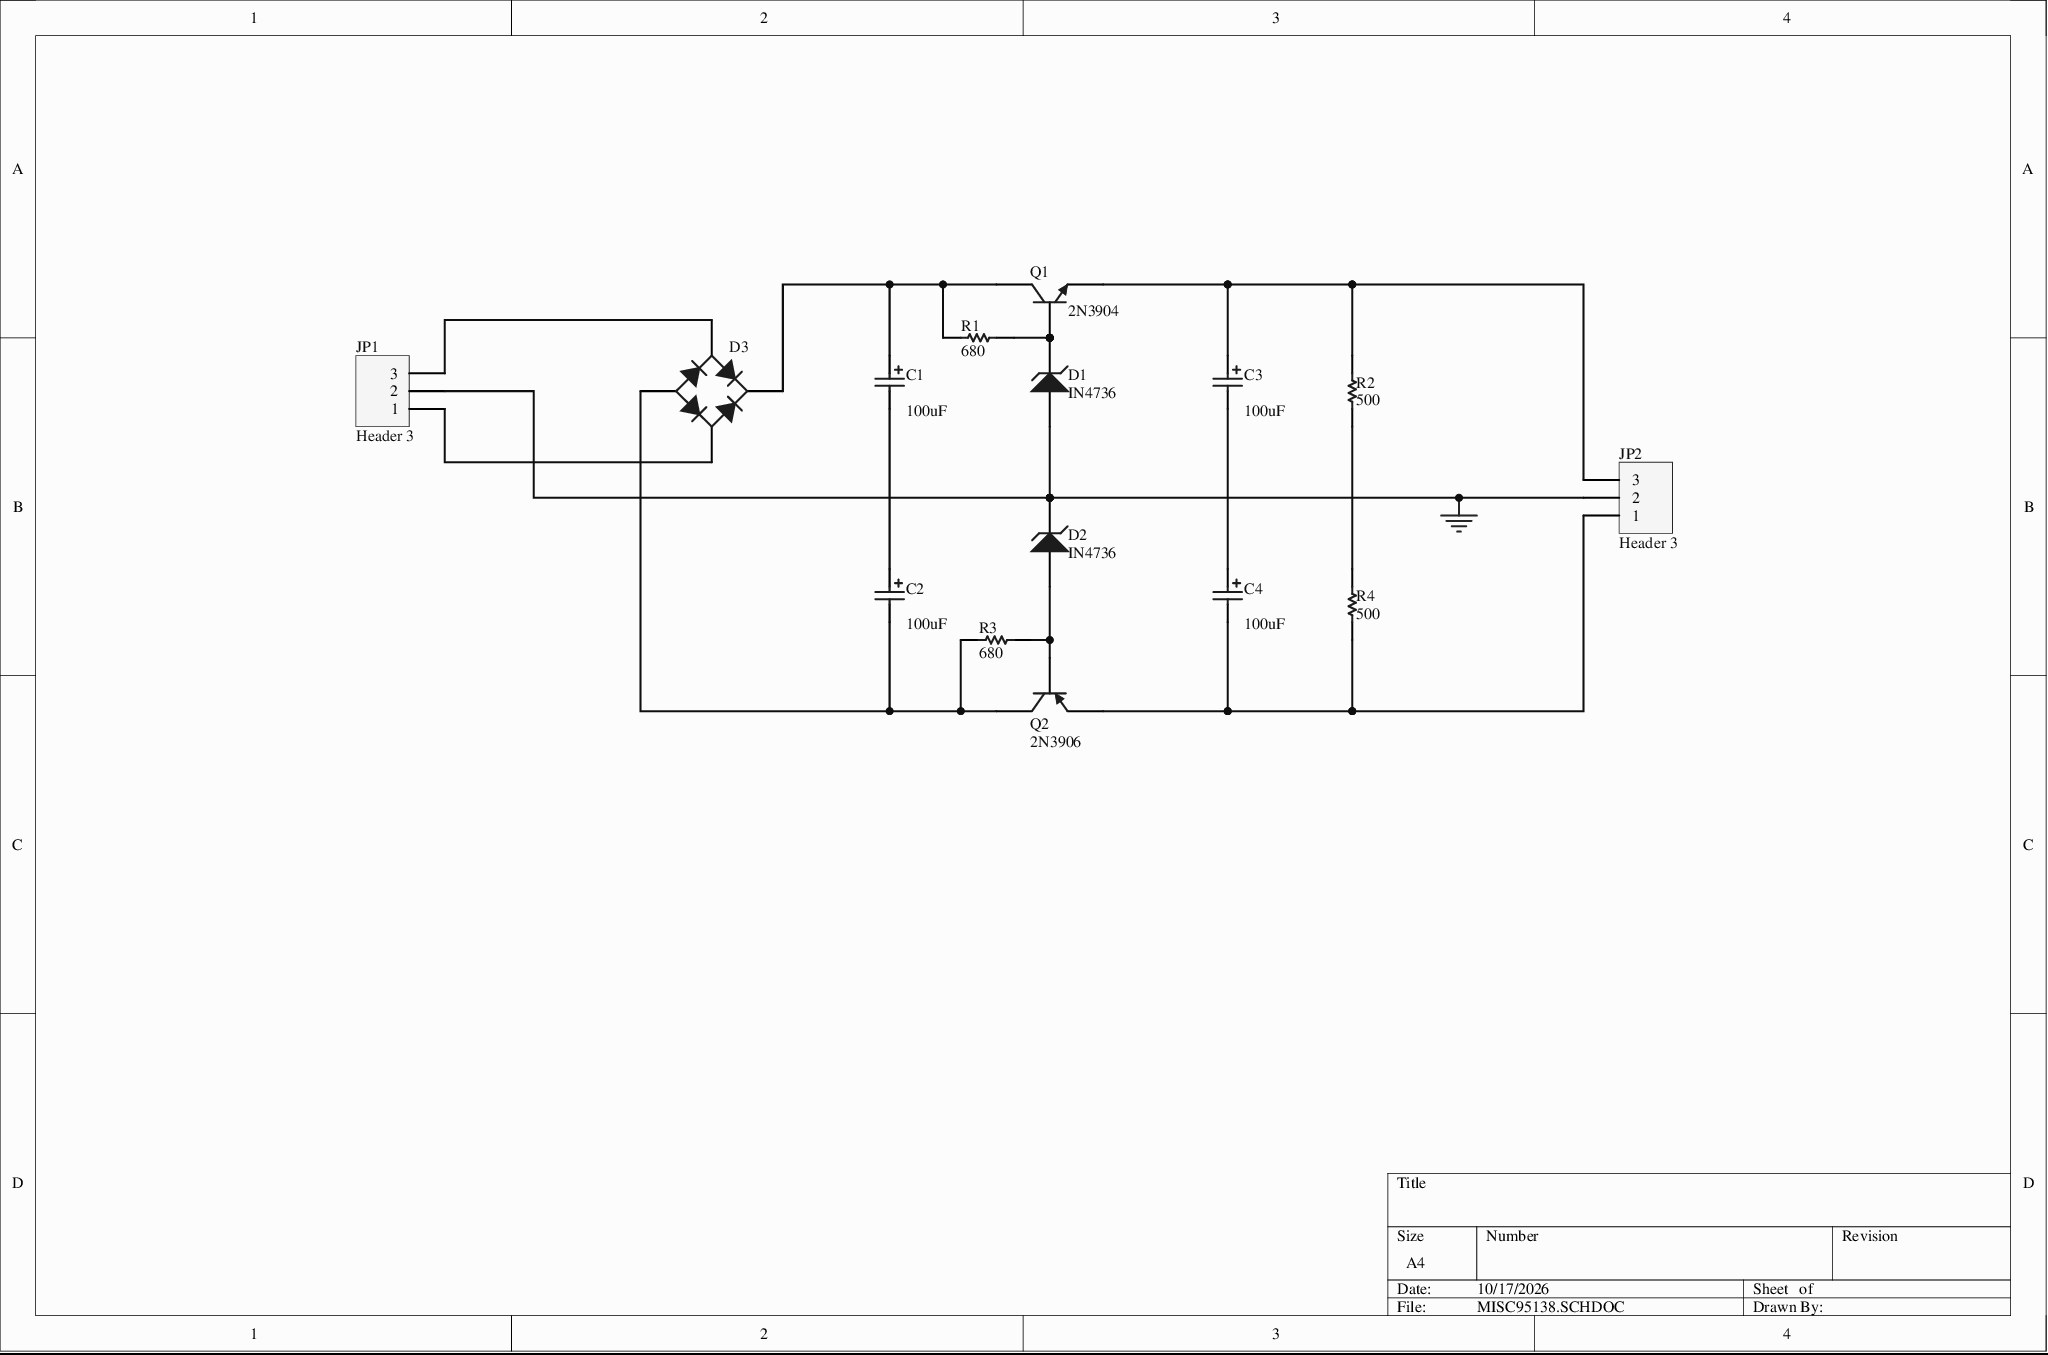
[diagram p0: MISC95138.SCHDOC]
# Altium project MISC95138.PRJPCB
1 sheet, 15 parts. Net scope: global (net labels, ports and power ports of the same name join across sheets).
Board file: MISC95138.PCBDOC

## Sheet MISC95138.SCHDOC
size A4

### Parts
C1  value 100uF  [RB7.6-15]  (hidden comment: Cap Pol1)
C2  value 100uF  [RB7.6-15]  (hidden comment: Cap Pol1)
C3  value 100uF  [RB7.6-15]  (hidden comment: Cap Pol1)
C4  value 100uF  [RB7.6-15]  (hidden comment: Cap Pol1)
D1  IN4736  [DIODE-0.7]
D2  IN4736  [DIODE-0.7]
D3  Bridge1  [E-BIP-P4/D10]  (value not drawn)
JP1  Header 3  [HDR1X3]
JP2  Header 3  [HDR1X3]
Q1  2N3904  [BCY-W3/E4]
Q2  2N3906  [BCY-W3/E4]
R1  value 680  [AXIAL-0.3]  (hidden comment: Res1)
R2  value 500  [AXIAL-0.3]  (hidden comment: Res1)
R3  value 680  [AXIAL-0.3]  (hidden comment: Res1)
R4  value 500  [AXIAL-0.3]  (hidden comment: Res1)

### Nets
GND: D1.1(A) D2.2(K) JP1.2 JP2.2
NetC1_1: C1.1 D3.3(K) Q1.3(C) R1.1
NetC1_2: C1.2 C2.1
NetC2_2: C2.2 D3.1(A) Q2.3(C) R3.1
NetC3_1: C3.1 JP2.3 Q1.1(E) R2.2
NetC3_2: C3.2 C4.1
NetC4_2: C4.2 JP2.1 Q2.1(E) R4.1
NetD1_2: D1.2(K) Q1.2(B) R1.2
NetD2_1: D2.1(A) Q2.2(B) R3.2
NetD3_2: D3.2(C) JP1.3
NetD3_4: D3.4(C) JP1.1
NetR2_1: R2.1 R4.2

### Library data of the parts
C1-C4 = Cap Pol1: Polarized Capacitor (Radial); Published: 8-Jun-2000; Revision: July-2002: Re-released for DXP Platform.; Publisher: Altium Limited
D1 D2 = D Zener: Zener Diode; Published: 8-Jun-2000; Revision: July-2002: Re-released for DXP Platform.; Publisher: Altium Limited
D3 = Bridge1: Full Wave Diode Bridge; Published: 8-Jun-2000; Revision: July-2002: Re-released for DXP Platform.; Publisher: Altium Limited
JP1 JP2 = Header 3: Header, 3-Pin; Revision: 17-Jul-2002: Re-released for DXP Platform.; Publisher: Altium Limited
Q1 = 2N3904: NPN General Purpose Amplifier; Revision 1: 11-Jul-2000: SIM Model Added.; Revision 2: 17-Jul-2002: Re-released for DXP Platform.; Revision 3: 15-Jan-2003: PCB Footprint 'BCY-W3/D4.7' replaced; Code - JEDEC: TO-92A; Published: 8-Jun-2000; Datasheet: Latest Revision: 1997; Package Reference: TO-92A; Publisher: Altium Limited
Q2 = 2N3906: PNP General Purpose Amplifier; Revision 1: 11-Jul-2000: SIM Model Added.; Revision 2: 17-Jul-2002: Re-released for DXP Platform.; Revision 3: 15-Jan-2003: PCB Footprint 'BCY-W3/D4.7' replaced; Code - JEDEC: TO-92A; Published: 8-Jun-2000; Datasheet: Latest Revision: 1997; Package Reference: TO-92A; Publisher: Altium Limited
R1-R4 = Res1: Resistor; Published: 8-Jun-2000; Revision: July-2002: Re-released for DXP Platform.; Publisher: Altium Limited